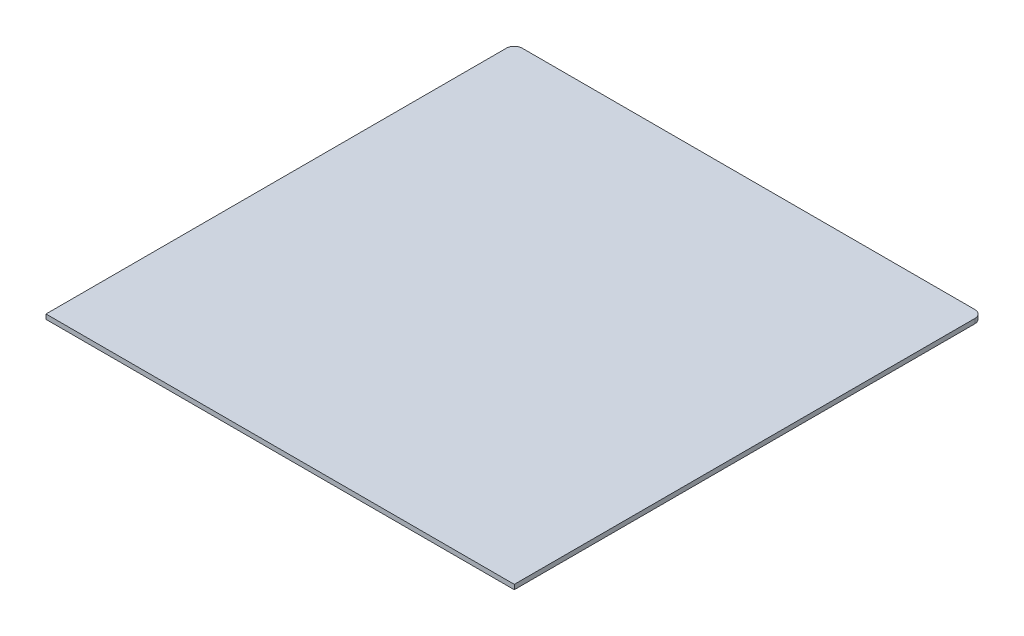
SolidWorks part; units mm, degrees
ref_plane "Front Plane" through (0, 0, 0) normal (0, 0, 1) x (1, 0, 0)
ref_plane "Top Plane" through (0, 0, 0) normal (0, 1, 0) x (1, 0, 0)
ref_plane "Right Plane" through (0, 0, 0) normal (1, 0, 0) x (0, 0, -1)
sketch "Sketch1" plane through (0, 0, 0) normal (0, 1, 0) x (1, 0, 0)
  line L1 (-150, -150) -> (150, -150)
  line L2 (-150, -150) -> (-150, 145)
  line L3 (-145, 150) -> (145, 150)
  line L4 (150, -150) -> (150, 145)
  line L5 (-150, -150) -> (150, 150) construction
  line L6 (-150, 150) -> (150, -150) construction
  arc A0 (145, 150) -> (150, 145) centre (145, 145) cw
  arc A1 (-150, 145) -> (-145, 150) centre (-145, 145) cw
  point P0 (0, 0)
  dimension "D3" = 5
  dimension "D1" = 300
  dimension "D2" = 300
extrude "Boss-Extrude1" add sketch "Sketch1" along normal blind 3
